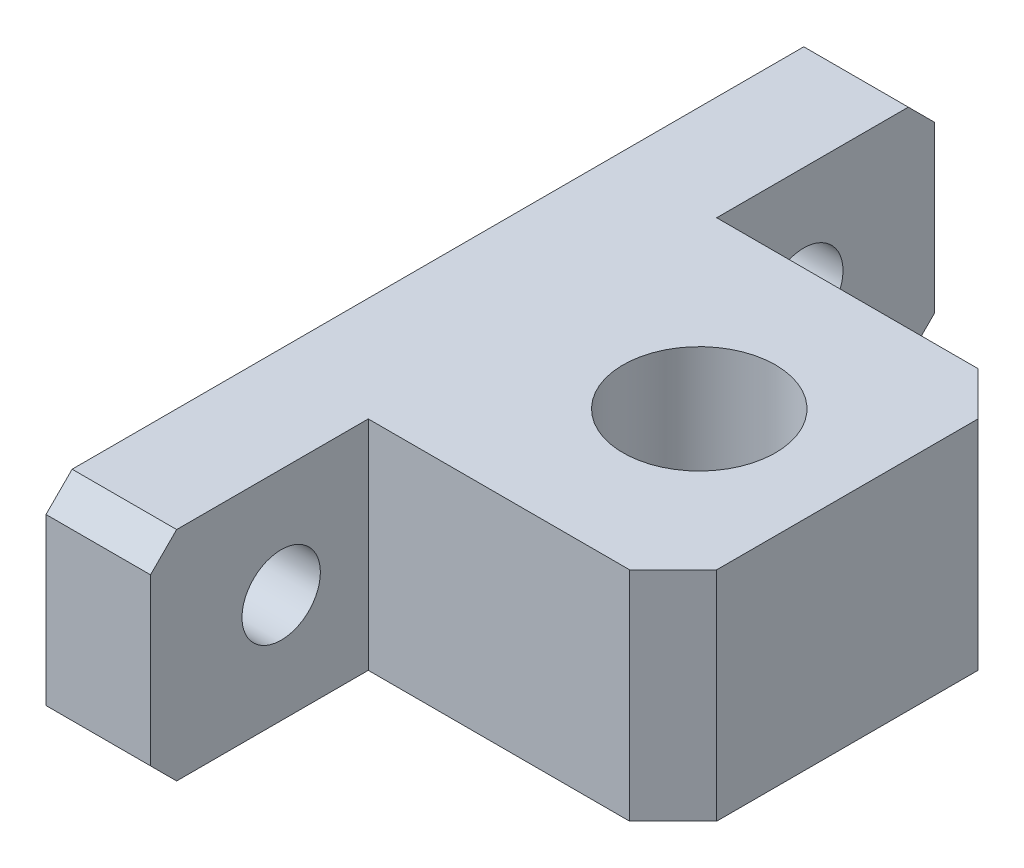
SolidWorks part; units mm, degrees
ref_plane "前视基准面" through (0, 0, 0) normal (0, 0, 1) x (1, 0, 0)
ref_plane "上视基准面" through (0, 0, 0) normal (0, 1, 0) x (1, 0, 0)
ref_plane "右视基准面" through (0, 0, 0) normal (1, 0, 0) x (0, 0, -1)
sketch "草图1" plane through (0, 0, 0) normal (1, 0, 0) x (0, 0, -1)
  line L1 (-45, 12.5) -> (45, 12.5)
  line L2 (-45, 12.5) -> (-45, -12.5)
  line L3 (-45, -12.5) -> (45, -12.5)
  line L4 (45, 12.5) -> (45, -12.5)
  line L5 (-45, 12.5) -> (45, -12.5) construction
  line L6 (-45, -12.5) -> (45, 12.5) construction
  point P0 (0, 0)
  dimension "D1" = 90
  dimension "D2" = 25
extrude "凸台-拉伸1" add sketch "草图1" along normal blind 12
sketch "草图2" plane through (12, 0, 0) normal (1, 0, 0) x (0, 0, -1)
  line L1 (-20, 12.5) -> (20, 12.5)
  line L2 (-20, 12.5) -> (-20, -12.5)
  line L3 (-20, -12.5) -> (20, -12.5)
  line L4 (20, 12.5) -> (20, -12.5)
  line L5 (-20, 12.5) -> (20, -12.5) construction
  line L6 (-20, -12.5) -> (20, 12.5) construction
  point P0 (0, 0)
  dimension "D1" = 40
  dimension "D2" = 25
extrude "凸台-拉伸2" add sketch "草图2" along normal blind 35
hole_wizard "M20 螺纹孔1" positions "草图3" profile "草图4" tap size "M20" standard "GB" end condition through all
sketch "草图3" plane through (0, -12.5, 0) normal (0, -1, 0) x (-1, 0, 0)
  line L0 (0, -45) -> (0, 45) construction
  point P0 (-30, 0)
  dimension "D1" = 30
sketch "草图4" plane through (30, -12.5, 0) normal (1, 0, 0) x (0, 0, -1)
  line L0 (0, 0) -> (0, 25)
  line L1 (0, 25) -> (8.75, 25)
  line L2 (8.75, 25) -> (8.75, 0)
  line L5 (8.75, 0) -> (0, 0)
  line L11 (0, -6.35) -> (0, 107.95) construction
  dimension "通孔螺纹孔钻头直径" = 17.5
  dimension "通孔螺纹孔钻头深度" = 25
cosmetic thread "孔螺蚊线1" parameters "D2"=20
hole_wizard "Ø9.0 (9) 直径孔1" positions "草图5" profile "草图6" hole size "Ø9.0" standard "GB" end condition through all
sketch "草图5" plane through (12, 0, 0) normal (1, 0, 0) x (0, 0, -1)
  line L0 (0, 47.7647) -> (0, 0) construction
  line L1 (0, 0) -> (53.9093, 0) construction
  point P4 (-30, 0)
  point P6 (30, 0)
  dimension "D1" = 60
sketch "草图6" plane through (12, 0, 30) normal (0, 1, 0) x (0, 0, -1)
  line L0 (0, 0) -> (0, 12)
  line L1 (0, 12) -> (4.5, 12)
  line L2 (4.5, 12) -> (4.5, 0)
  line L5 (4.5, 0) -> (0, 0)
  line L11 (0, -6.35) -> (0, 107.95) construction
  dimension "通孔孔直径" = 9
  dimension "通孔孔深度" = 12
chamfer "倒角1" distance 5 angle 45 2 edges at (47, 0, -20) (47, 0, 20)
chamfer "倒角2" distance 3 angle 45 4 edges at (6, 12.5, -45) (6, -12.5, -45) (6, 12.5, 45) (6, -12.5, 45)
